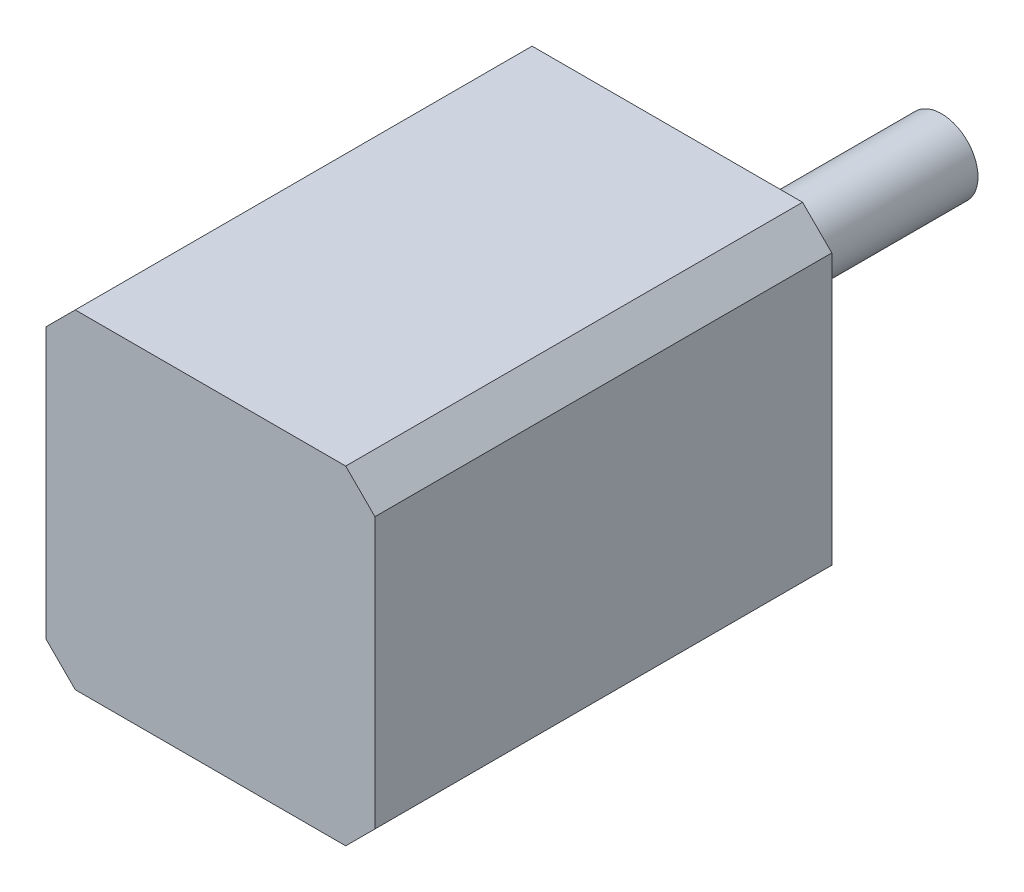
from build123d import *

# Parameters (mm, degrees)
SKETCH1_R           = 20
BOSS_EXTRUDE1_DEPTH = 140
SKETCH2_R           = 45
BOSS_EXTRUDE2_DEPTH = 10
SKETCH3_W           = 180
SKETCH3_H           = 180
BOSS_EXTRUDE3_DEPTH = 250
CHAMFER1_SIZE       = 16


with BuildPart() as part:
    # Sketch1 → Boss-Extrude1 (new body)
    with BuildSketch(Plane.XY):
        Circle(SKETCH1_R)
    extrude(amount=BOSS_EXTRUDE1_DEPTH)

    # Sketch2 → Boss-Extrude2 (add)
    with BuildSketch(Plane.XY.offset(140)):
        Circle(SKETCH2_R)
    extrude(amount=BOSS_EXTRUDE2_DEPTH)

    # Sketch3 → Boss-Extrude3 (add)
    with BuildSketch(Plane.XY.offset(150)):
        Rectangle(SKETCH3_W, SKETCH3_H)
    extrude(amount=BOSS_EXTRUDE3_DEPTH)

    # Chamfer1
    chamfer1_edges = [part.edges().sort_by_distance(p)[0] for p in [
        (90, -90, 275),
        (90, 90, 275),
        (-90, 90, 275),
        (-90, -90, 275),
    ]]
    chamfer(chamfer1_edges, length=CHAMFER1_SIZE)


solid = part.part
